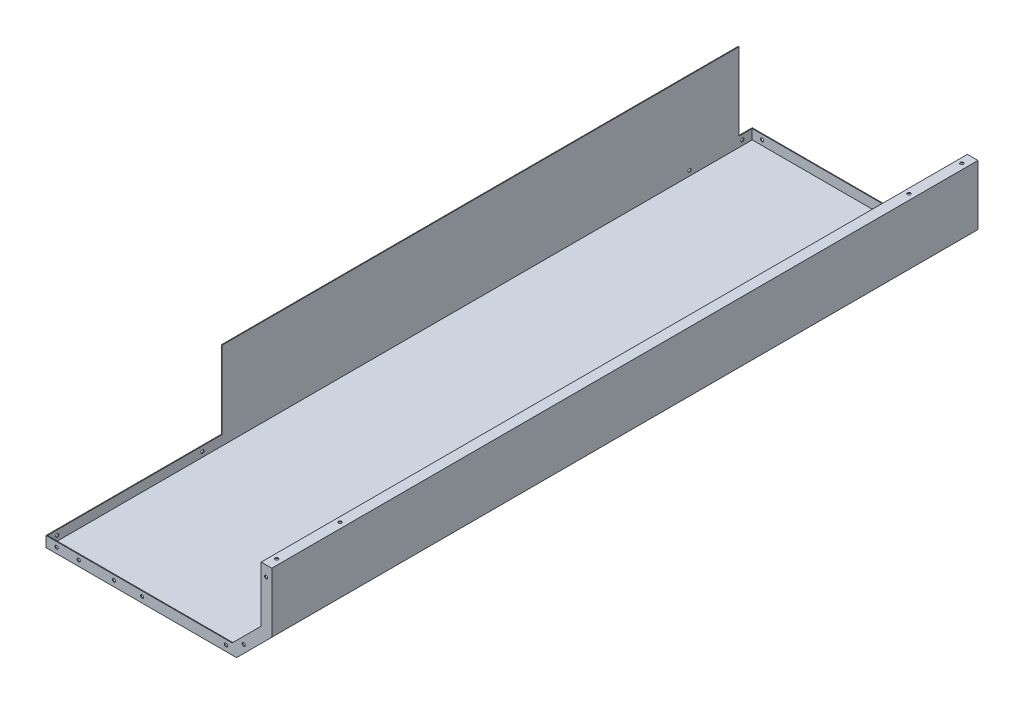
from build123d import *

# Parameters (mm, degrees)
EXTRUDE_1_DEPTH     = 2005
EXTRUDE_1_2_DEPTH   = 28
SKETCH_5_W          = 2
SKETCH_5_H          = 139.764501987
EXTRUDE_2_DEPTH     = 28
SKETCH_6_W          = 540.171572875
SKETCH_6_H          = 2
EXTRUDE_3_DEPTH     = 28
SKETCH_7_W          = 2
SKETCH_7_H          = 2005
EXTRUDE_4_DEPTH     = 28
SKETCH_8_W          = 2
SKETCH_8_H          = 1467
EXTRUDE_5_DEPTH     = 220
SKETCH_9_R          = 4.5
CUT_EXTRUDE_1_DEPTH = 10
SKETCH_11_R         = 4.5
CUT_EXTRUDE_2_DEPTH = 10
SKETCH_12_R         = 4.5
CUT_EXTRUDE_3_DEPTH = 116
SKETCH_13_R         = 4.5
CUT_EXTRUDE_4_DEPTH = 63
SKETCH_14_R         = 4.5
CUT_EXTRUDE_5_DEPTH = 72
CUT_EXTRUDE_START   = -2
SKETCH_15_R         = 4.5
CUT_EXTRUDE_6_DEPTH = 2


with BuildPart() as part:
    # 草图1 → Extrude 1 (new body)
    with BuildSketch(Plane.XY):
        Polygon((0, 0), (541, 0), (641, 100), (641, 270), (639, 270), (639, 100.828427125), (540.171572875, 2), (0, 2), align=None)
    extrude(amount=EXTRUDE_1_DEPTH)

    # 草图4 → Extrude 1 2 (add)
    with BuildSketch(Plane.ZY.offset(-639)):
        Polygon((0, 100.828427125), (0, 270), (2005, 270), (2005, 100.828427125), (2003, 100.828427125), (2003, 268), (2, 268), (2, 100.828427125), align=None)
    extrude(amount=EXTRUDE_1_2_DEPTH)

    # 草图5 → 凸台-拉伸2 (add)
    with BuildSketch(Plane(origin=(269.085786438, -269.085786438, 0), x_dir=(0, 0, 1), z_dir=(-0.7071067811865476, 0.7071067811865476, 0))):
        with Locations((1, 453.255446741)):
            Rectangle(SKETCH_5_W, SKETCH_5_H)
        with Locations((2004, 453.255446741)):
            Rectangle(SKETCH_5_W, SKETCH_5_H)
    extrude(amount=EXTRUDE_2_DEPTH)

    # 草图6 → 凸台-拉伸3 (add)
    with BuildSketch(Plane(origin=(0, 2, 0), x_dir=(1, 0, 0), z_dir=(0, 1, 0))):
        with Locations((270.085786438, -1)):
            Rectangle(SKETCH_6_W, SKETCH_6_H)
        with Locations((270.085786438, -2004)):
            Rectangle(SKETCH_6_W, SKETCH_6_H)
    extrude(amount=EXTRUDE_3_DEPTH)

    # 草图7 → 凸台-拉伸4 (add)
    with BuildSketch(Plane(origin=(0, 2, 0), x_dir=(1, 0, 0), z_dir=(0, 1, 0))):
        with Locations((1, -1002.5)):
            Rectangle(SKETCH_7_W, SKETCH_7_H)
    extrude(amount=EXTRUDE_4_DEPTH)

    # 草图8 → 凸台-拉伸5 (add)
    with BuildSketch(Plane(origin=(0, 30, 0), x_dir=(1, 0, 0), z_dir=(0, 1, 0))):
        with Locations((1, -773.5)):
            Rectangle(SKETCH_8_W, SKETCH_8_H)
    extrude(amount=EXTRUDE_5_DEPTH)

    # 草图9 → 切除-拉伸1 (cut)
    with BuildSketch(Plane.XY.offset(2)):
        with Locations((625, 240)):
            Circle(SKETCH_9_R)
        with Locations((30, 16)):
            Circle(SKETCH_9_R)
        with Locations((431, 16)):
            Circle(SKETCH_9_R)
        with Locations((625, 140)):
            Circle(SKETCH_9_R)
    extrude(amount=-CUT_EXTRUDE_1_DEPTH, mode=Mode.SUBTRACT)

    # 草图11 → 切除-拉伸2 (cut)
    with BuildSketch(Plane.XZ.offset(-268)):
        with Locations(Location((625, 30, 0), (0, 0, 270))):
            Circle(SKETCH_11_R)
        with Locations(Location((625, 180, 0), (0, 0, 270))):
            Circle(SKETCH_11_R)
    extrude(amount=-CUT_EXTRUDE_2_DEPTH, mode=Mode.SUBTRACT)

    # 草图12 → 切除-拉伸3 (cut)
    with BuildSketch(Plane(origin=(2, 0, 0), x_dir=(0, 0, -1), z_dir=(1, 0, 0))):
        with Locations((-30, 16)):
            Circle(SKETCH_12_R)
        with Locations((-180, 16)):
            Circle(SKETCH_12_R)
    extrude(amount=-CUT_EXTRUDE_3_DEPTH, mode=Mode.SUBTRACT)

    # 草图13 → 切除-拉伸4 (cut)
    with BuildSketch(Plane.XZ.offset(-268)):
        with Locations(Location((625, 1975, 0), (0, 0, 270))):
            Circle(SKETCH_13_R)
        with Locations(Location((625, 1795, 0), (0, 0, 270))):
            Circle(SKETCH_13_R)
    extrude(amount=-CUT_EXTRUDE_4_DEPTH, mode=Mode.SUBTRACT)

    # 草图14 → 切除-拉伸5 (cut)
    with BuildSketch(Plane(origin=(2, 0, 0), x_dir=(0, 0, -1), z_dir=(1, 0, 0))):
        with Locations((-1975, 16)):
            Circle(SKETCH_14_R)
        with Locations((-1563, 16)):
            Circle(SKETCH_14_R)
    extrude(amount=-CUT_EXTRUDE_5_DEPTH, mode=Mode.SUBTRACT)

    # 草图15 → 切除-拉伸6 (cut)
    with BuildSketch(Plane(origin=(0, 0, 2003), x_dir=(-1, 0, 0), z_dir=(0, 0, -1)).offset(CUT_EXTRUDE_START)):
        with Locations(Location((-625, 240, 0), (0, 0, 180))):
            Circle(SKETCH_15_R)
        with Locations((-561.360389693, 42.987806691)):
            Circle(SKETCH_15_R)
        with Locations(Location((-30, 16, 0), (0, 0, 180))):
            Circle(SKETCH_15_R)
        with Locations((-511, 16)):
            Circle(SKETCH_15_R)
        with Locations((-273, 16)):
            Circle(SKETCH_15_R)
        with Locations((-193, 16)):
            Circle(SKETCH_15_R)
        with Locations((-93, 16)):
            Circle(SKETCH_15_R)
    extrude(amount=CUT_EXTRUDE_6_DEPTH, mode=Mode.SUBTRACT)


solid = part.part
